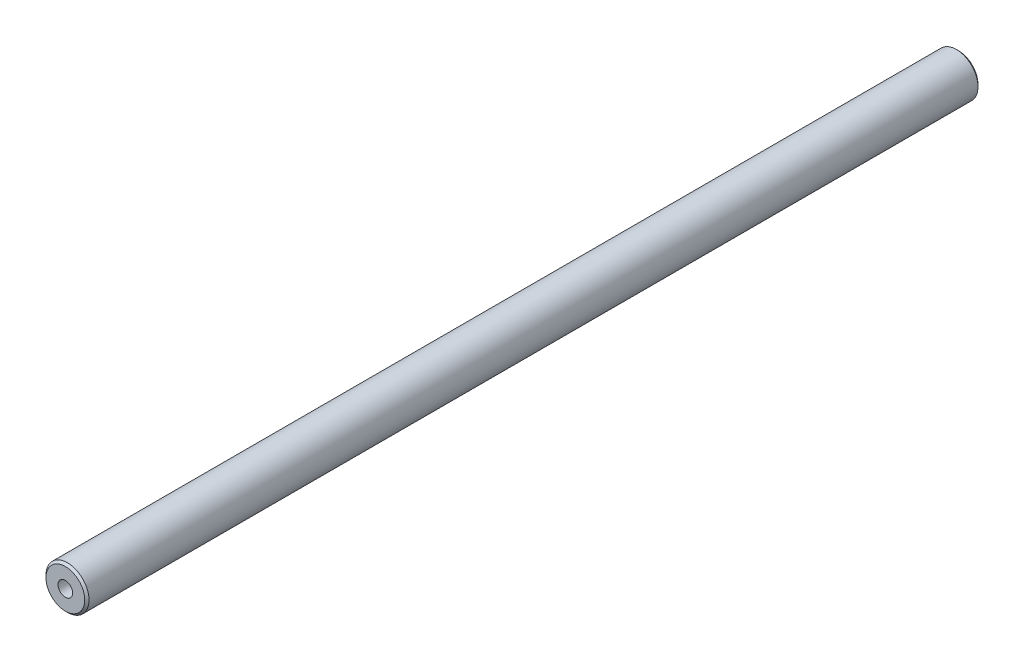
from build123d import *

# Parameters (mm, degrees)
SKETCH_1_R             = 10
EXTRUDE_1_DEPTH        = 415
HOLE_WIZARD_M8_1_D     = 6.8
HOLE_WIZARD_M8_1_DEPTH = 22.25
HOLE_WIZARD_M8_1_TIP   = 2.042926105
CHAMFER_1_SIZE         = 1
HOLE_WIZARD_M8_2_D     = 6.8
HOLE_WIZARD_M8_2_DEPTH = 22.25
HOLE_WIZARD_M8_2_TIP   = 2.042926105


with BuildPart() as part:
    # 草图1 → 凸台-拉伸1 (new body)
    with BuildSketch(Plane.XY):
        Circle(SKETCH_1_R)
    extrude(amount=EXTRUDE_1_DEPTH)

    # M8 螺纹孔1
    with Locations(Plane.XY.offset(415)):
        with Locations((0, 0)):
            Hole(HOLE_WIZARD_M8_1_D / 2, depth=HOLE_WIZARD_M8_1_DEPTH)
            with Locations((0, 0, -(HOLE_WIZARD_M8_1_DEPTH + HOLE_WIZARD_M8_1_TIP / 2))):  # 118° drill point
                Cone(0, HOLE_WIZARD_M8_1_D / 2, HOLE_WIZARD_M8_1_TIP, mode=Mode.SUBTRACT)

    # 倒角1
    chamfer_1_edges = [part.edges().sort_by_distance(p)[0] for p in [
        (-10, 0, 0),
        (-10, 0, 415),
    ]]
    chamfer(chamfer_1_edges, length=CHAMFER_1_SIZE)

    # M8 螺纹孔2
    with Locations(Plane(origin=(0, 0, 0), x_dir=(-1, 0, 0), z_dir=(0, 0, -1))):
        with Locations((0, 0)):
            Hole(HOLE_WIZARD_M8_2_D / 2, depth=HOLE_WIZARD_M8_2_DEPTH)
            with Locations((0, 0, -(HOLE_WIZARD_M8_2_DEPTH + HOLE_WIZARD_M8_2_TIP / 2))):  # 118° drill point
                Cone(0, HOLE_WIZARD_M8_2_D / 2, HOLE_WIZARD_M8_2_TIP, mode=Mode.SUBTRACT)


solid = part.part
